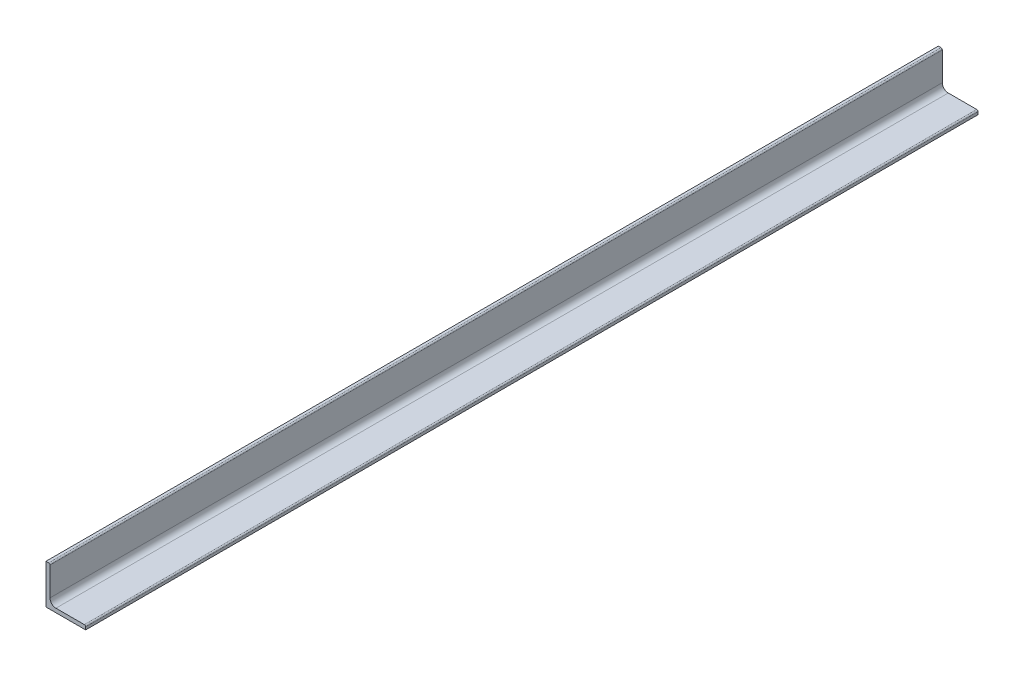
from build123d import *

# Parameters (mm, degrees)
BOSS_EXTRUDE1_DEPTH = 337.5


with BuildPart() as part:
    # Sketch1 → Boss-Extrude1 (new, symmetric)
    with BuildSketch(Plane.XY):
        with BuildLine():
            Line((0, 0), (0, 30))
            Line((0, 30), (2, 30))
            ThreePointArc((2, 30), (2.707106781, 29.707106781), (3, 29))
            Line((3, 29), (3, 7.5))
            ThreePointArc((3, 7.5), (4.318019485, 4.318019485), (7.5, 3))
            Line((7.5, 3), (29, 3))
            ThreePointArc((29, 3), (29.707106781, 2.707106781), (30, 2))
            Line((30, 2), (30, 0))
            Line((30, 0), (0, 0))
        make_face()
    extrude(amount=BOSS_EXTRUDE1_DEPTH, both=True)


solid = part.part
